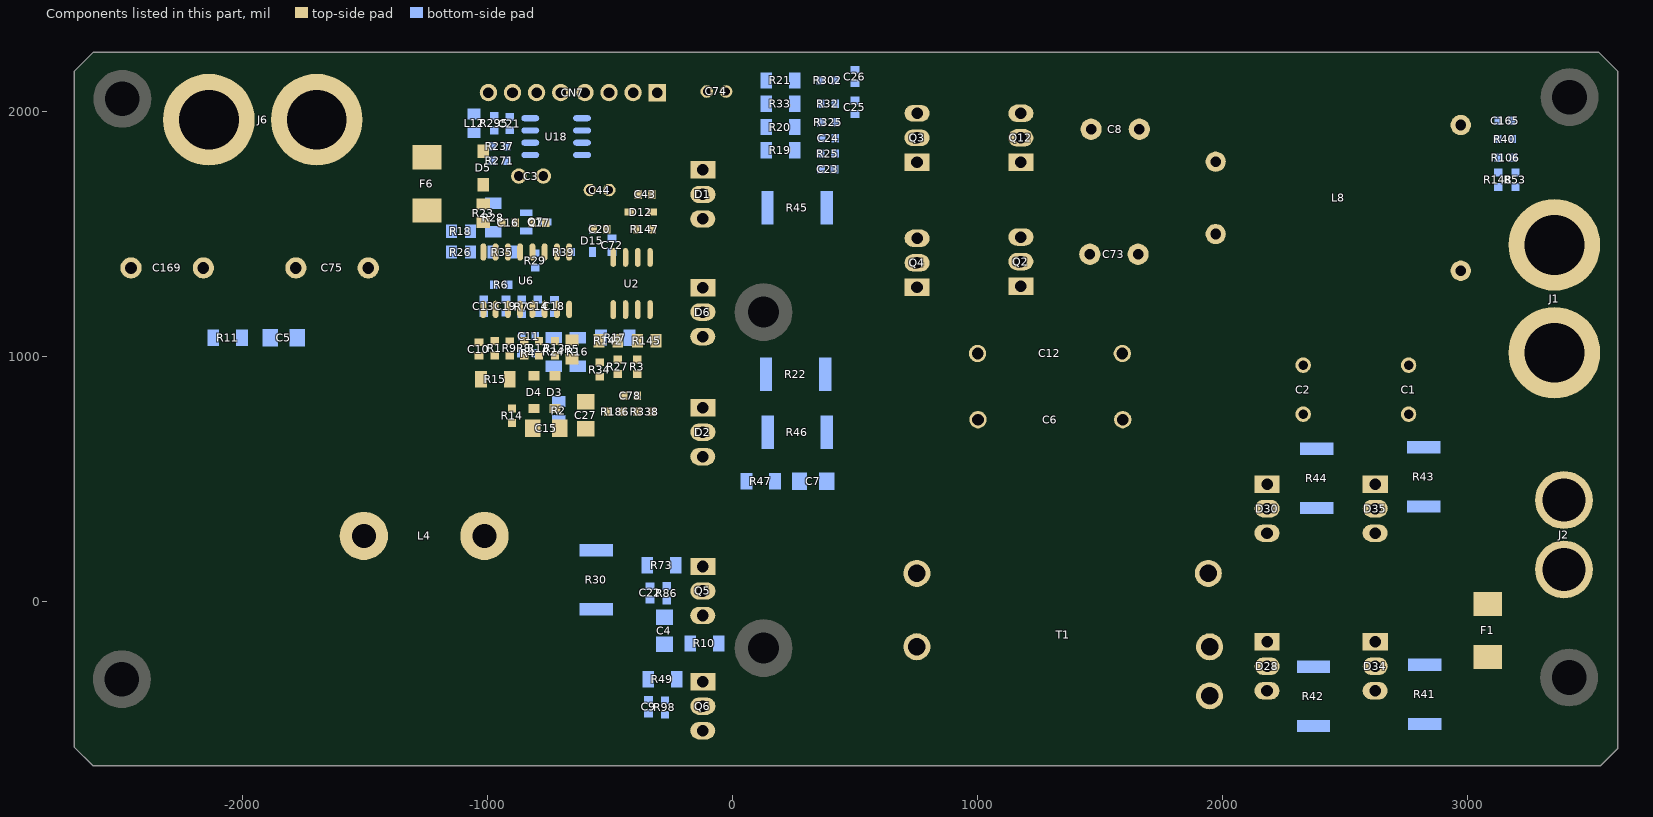
[diagram p0: the components of this part, seen from the top]
# Altium PCB MISC89356.PcbDoc (part 3 of 3)
Units mil, origin at the board's own origin, x right, y up, seen from the top; angles counter-clockwise.
Board outline 6299.21 x 2912.91 mil, 4 copper layers (Top Layer, GND02, PWR03, Bottom Layer); 128 components, 68 nets, 313 pads, 200 vias.

## Polygon pours and split planes (outlines as drawn) (continued)
GND on GND02 "Bottom Layer-No Net 2" (solid, remove dead copper, pour order 1001): -1142.15,2154.47 -1142.15,779.66 -897.15,527.35 -877.15,506.76 -877.15,-239.86 -877.15,-569.4 -897.15,-590 -2607.15,-590 -2687.15,-507.61 -2687.15,2159.61 -2607.15,2242 -1152.15,2242 -1147.15,2236.85 -1142.15,2231.7 -1142.15,2154.47
BAT- on GND02 "BottomLayer-No Net" (solid, remove dead copper, pour order 1004): -653,89 -653,72 -653,-517 -607,-563 -591,-579 -132,-579 557,-579 619,-517 654,-482 654,-413 654,779 675,800 683,808 865,808 1746,808 1813,741 1854,700 1854,29 1854,-451 1877,-474 1927,-524 2014,-524 3513,-524 3555,-482 3581,-456 3581,-411 3581,1604 3545,1640 3523,1662 3447,1662 2997,1662 2954,1619 2932,1597 2932,1455 2932,1188 2870,1126 2862,1118 2796,1118 1825,1118 1778,1165 1758,1185 1758,1326 1758,2097 1688,2167 1668,2187 1585,2187 292,2187 239,2134 227,2122 227,2090 227,1802 209,1784 204,1779 142,1779 -140,1779 -204,1715 -231,1688 -231,1584 -231,212 -254,189 -256,191 -533,191 -600,191 -639,152 -653,138 -653,90
GND on GND02 "BottomLayer-No Net" (solid, remove dead copper, pour order 1006): -1061,2137 -1061,838 -807,584 -684,461 -684,300 -684,293 -664,273 -649,258 -585,258 -364,258 -344,278 -339,283 -339,743 -339,815 -315,839 -298,856 -298,902 -298,1836 -267,1867 -259,1875 -36,1875 24,1875 58,1909 69,1920 69,1975 69,2161 44,2186 23,2207 -30,2207 -994,2207 -1062,2139
NetD30_1 on PWR03 "BottomLayer-No Net" (solid, remove dead copper, pour order 1004): 1869,318 1869,93 1898,64 1904,58 1917,45 2667,45 2746,45 2780,79 2805,104 2805,211 2805,555 2748,612 2723,637 2651,637 1943,637 1893,587 1869,563 1869,318
NetD28_1 on PWR03 "BottomLayer-No Net" (solid, remove dead copper, pour order 1003): 1883,-339 1883,-461 1898,-476 1913,-491 1942,-491 2742,-491 2767,-466 2777,-456 2777,-389 2777,-84 2750,-57 2730,-37 2681,-37 2104,-37 2053,-88 2043,-98 2043,-165 2043,-234 2019,-258 1998,-279 1945,-279 1899,-279 1891,-287 1883,-295 1883,-339
GND on PWR03 "Bottom Layer-No Net 2" (solid, remove dead copper, pour order 1006): -1142.15,2154.74 -1142.15,784.31 -897.15,532.8 -877.15,512.27 -877.15,-231.97 -877.15,-560.47 -897.15,-581 -2607.15,-581 -2687.15,-498.88 -2687.15,2159.88 -2607.15,2242 -1152.15,2242 -1147.15,2236.87 -1142.15,2231.73 -1142.15,2154.74
BAT- on PWR03 "BottomLayer-No Net" (solid, remove dead copper, pour order 1008): -683,-31 -683,-523 -651,-555 -597,-609 -216,-609 577,-609 623,-563 649,-537 649,-367 649,715 719,785 800,866 2364,866 2839,866 2928,777 3003,702 3003,517 3003,380 3044,339 3122,261 3342,261 3476,261 3522,307 3570,355 3570,495 3570,1785 3527,1828 3514,1841 3337,1841 3118,1841 3085,1808 3068,1791 3068,1535 3068,1129 3048,1109 3040,1101 2835,1101 1871,1101 1843,1129 1829,1143 1829,1369 1829,2108 1773,2164 1749,2188 1660,2188 260,2188 241,2169 233,2161 233,2113 233,1865 209,1841 177,1809 -31,1809 -166,1809 -181,1794 -224,1751 -224,1725 -224,181 -267,138 -313,92 -538,92 -636,92 -672,56 -683,45 -683,-30
GND on PWR03 "BottomLayer-No Net" (solid, remove dead copper, pour order 1009): -1060,2162 -1060,851 -723,514 -713,504 -713,439 -713,299 -679,265 -662,248 -590,248 -366,248 -343,271 -343,727 -343,835 -308,870 -298,880 -298,918 -298,1817 -248,1867 -232,1883 -70,1883 44,1883 78,1917 86,1925 86,1988 86,2158 53,2191 36,2208 -20,2208 -1022,2208 -1056,2174 -1060,2170 -1060,2162
NetC1_1 on Bottom Layer "BottomLayer-No Net" (solid, remove dead copper, pour order 1006): 2212,803 2212,634 2242,604 2263,583 2348,583 2877,583 2922,538 2968,492 2968,-81 2968,-368 2916,-420 2901,-435 2558,-435 2314,-435 2300,-449 2292,-457 2292,-482 2292,-550 2297,-555 2314,-572 2347,-572 3041,-572 3084,-529 3172,-441 3172,-84 3172,751 3112,811 3070,853 2740,853 2231,853 2212,834 2212,804
NetD30_2 on Bottom Layer "BOTTOM-No Net" (solid, remove dead copper, pour order 1004): 2403.36,183 2091.47,183 2074.15,204.6 2074.15,415.2 2082.81,426 2455.34,426 2464,415.2 2464,199.2 2455.34,188.4 2451,183 2403.36,183
LLC_I on Bottom Layer "BottomLayer-No Net" (solid, remove dead copper, pour order 1005): 569,517 569,497 569,97 604,62 617,49 688,49 786,49 799,62 809,72 809,122 809,574 862,627 875,640 967,640 1038,640 1061,663 1085,687 1085,732 1085,1061 1072,1074 1050,1096 992,1096 765,1096 689,1020 569,900 569,517
NetD35_2 on Bottom Layer "BOTTOM-No Net" (solid, remove dead copper, pour order 1005): 2567.53,419 2884.06,419 2907,393.4 2907,183.48 2888.65,163 2553.76,163 2540,178.36 2540,408.76 2549.18,419 2567.53,419
NetD28_2 on Bottom Layer "BOTTOM-No Net" (solid, remove dead copper, pour order 1006): 2053.85,-38 2423.85,-38 2443.85,-58 2443.85,-288 2428.85,-303 2068.85,-303 2038.85,-273 2038.85,-53
NetD34_2 on Bottom Layer "BOTTOM-No Net" (solid, remove dead copper, pour order 1007): 2566.29,-45 2886.23,-45 2904,-65 2904,-280 2890.67,-295 2886.23,-300 2597.39,-300 2530.74,-300 2521.85,-290 2521.85,-60 2535.18,-45 2566.29,-45
NetD1_2 on Bottom Layer "Bottom Layer-No Net 2" (solid, remove dead copper, pour order 1008): 187.85,1472 187.85,1702 172.85,1717 37.85,1717 22.85,1732 22.85,1827 2.85,1847 -222.15,1847 -232.15,1837 -232.15,1442 -212.15,1422 172.85,1422 187.85,1437 187.85,1472
PV+ on Bottom Layer "Bottom Layer-No Net 2" (solid, remove dead copper, pour order 1009): -1247.15,2147 -1212.15,2112 -1212.15,1747 -1232.15,1727 -1847.15,1727 -1862.15,1742 -1862.15,2062 -1777.15,2147
GND on Bottom Layer "Bottom Layer-No Net 2" (solid, remove dead copper, pour order 1011): -466.15,349 -661.15,349 -676.15,334 -676.15,144 -656.15,124 -411.15,124 -396.15,139 -396.15,279 -466.15,349
GND on Bottom Layer "Bottom Layer-No Net 2" (solid, remove dead copper, pour order 1012): -1142.15,2154.47 -1142.15,779.66 -897.15,527.35 -877.15,506.76 -877.15,-239.86 -877.15,-569.4 -897.15,-590 -2607.15,-590 -2687.15,-507.61 -2687.15,2159.61 -2607.15,2242 -1152.15,2242 -1147.15,2236.85 -1142.15,2231.7 -1142.15,2154.47
BAT- on Bottom Layer "BottomLayer-No Net" (solid, remove dead copper, pour order 1012): -687,-31 -687,-507 -636,-558 -583,-611 -179,-611 -91,-611 -65,-585 -61,-581 -61,-545 -61,-511 -77,-495 -85,-487 -110,-487 -199,-487 -219,-467 -242,-444 -271,-444 -368,-444 -398,-414 -412,-400 -412,-239 -412,12 -425,25 -434,34 -465,34 -668,34 -681,21 -687,15 -687,-31
NetD6_2 on Bottom Layer "BottomLayer-No Net" (solid, remove dead copper, pour order 1013): -129,1231 -220,1231 -259,1192 -265,1186 -265,1107 -265,979 -227,941 -217,931 -77,931 -20,931 46,865 58,853 148,853 169,853 188,872 193,877 193,937 193,1005 172,1026 161,1037 114,1037 31,1037 -6,1074 -24,1092 -24,1185 -24,1200 -43,1219 -55,1231 -128,1231
NetD2_2 on Bottom Layer "BottomLayer-No Net" (solid, remove dead copper, pour order 1014): -253,831 -253,708 -231,686 -198,653 -124,653 6,653 37,622 54,605 115,605 167,605 182,620 200,638 200,679 200,788 178,810 176,812 126,812 44,812 -16,872 -34,890 -97,890 -227,890 -244,873 -253,864 -253,832
NetC7_2 on Bottom Layer "BottomLayer-No Net" (solid, remove dead copper, pour order 1015): 347,891 347,457 304,414 282,392 112,392 30,392 -50,472 -74,496 -150,496 -255,496 -325,566 -381,622 -381,955 -381,1107 -388,1114 -390,1116 -407,1116 -437,1116 -445,1108 -452,1101 -452,1068 -452,627 -283,458 -255,430 -145,430 -90,430 -25,365 22,318 213,318 386,318 449,381 490,422 490,596 490,983 567,1060 652,1145 796,1145 1499,1145 1541,1187 1571,1217 1571,1391 1571,2017 1560,2028 1545,2043 1502,2043 1344,2043 1334,2033 1302,2001 1302,1968 1302,1761 1278,1737 1232,1691 470,1691 379,1691 365,1677 347,1659 347,890

## Keep-outs
Keep-Out Layer:
  circle w10: c3414.78,2059.05 r70.87
  circle w10: c3412.93,-309.1 r70.87
  circle w10: c-2492.15,-315.95 r70.87
  circle w10: c-2490.3,2052.2 r70.87
  lines w25: -2687.15,-592 -2687.15,2164.17 -2608.41,2242.91 3533.33,2242.91 3612.07,2164.17 3612.07,-597.79 3539.85,-670 -2609.15,-670 -2687.15,-592

## Other copper
Top Layer:
  rectangle net NetD1_1: -231.15,-461 -21.15,-391
  rectangle net NetD1_1: -201.15,9 -26.15,79
  rectangle net NetD1_1: -207.15,762 -37.15,822
  rectangle net NetD1_1: -162.15,787 -82.15,857
  rectangle net NetD1_1: -162.54,527 -82.54,597
  rectangle net NetD1_1: -207.54,562 -37.54,622
  rectangle net NetD1_1: -207.15,1252 -37.15,1312
  rectangle net NetD1_1: -162.15,1277 -82.15,1347
  rectangle net NetD1_1: -162.54,1017 -82.54,1087
  rectangle net NetD1_1: -207.54,1052 -37.54,1112
  rectangle net NetD1_1: -207.54,1532 -37.54,1592
  rectangle net NetD1_1: -162.54,1497 -82.54,1567
  rectangle net NetD1_1: -162.15,1757 -82.15,1827
  rectangle net NetD1_1: -207.15,1732 -37.15,1792
  rectangle net T1H: 1095.46,1458 1265.46,1518
  rectangle net T1H: 1145.46,1488 1225.46,1558
  rectangle net T1H: 721.85,1482 801.85,1552
  rectangle net T1H: 671.85,1452 841.85,1512
  rectangle net T1H: 1935.85,1733 2005.85,1863
  rectangle net T1H: 1895.85,1763 2050.85,1833
  rectangle net NetL8_4: 700.85,-270 795.85,-90
  rectangle net NetL8_4: 661.85,-230 836.85,-135
  rectangle net NetL8_4: 1940.85,1438 2005.85,1568
  rectangle net NetL8_4: 1900.85,1472 2045.85,1532
  rectangle net GND: -633.71,1665 -583.71,1700
  rectangle net GND: -598.71,1630 -563.71,1730
  rectangle net +12V: -520.71,1384 -485.71,1431.2
  rectangle net +12V: -513.71,1659.53 -458.71,1700
  rectangle net +12V: -523.71,1625 -483.71,1730
  rectangle net GND: -2349,1857 -1947.15,2077
  rectangle net GND: -2277.15,1737 -1997.15,2182
  rectangle net PV+: -1901.15,1827 -1446.15,2113
  rectangle net PV+: -1809.15,1735 -1590.15,2177
  rectangle net PV+: -1382.15,1722 -1143.09,1854
  rectangle net PV+: -1297.15,1737 -1197.15,1927
  rectangle net PV-OVP: -1170.15,205 -863.15,340
  rectangle net PV-OVP: -1074.15,110 -946.15,410
  rectangle net PV-OVP: -1878.15,1329 -1686.15,1397
  rectangle net PV-OVP: -1813.15,1263 -1752.15,1449
  rectangle net PV-OVP: -2543.06,1329 -2358.15,1393
  rectangle net PV-OVP: -2485.15,1257 -2421.15,1463
  rectangle net PV-OVP: -1366.15,1561 -1142.15,1633
  rectangle net PV-OVP: -1293.15,1472 -1197.15,1577
  rectangle net NetC1_1: 2237.85,742 2417.85,792
  rectangle net NetC1_1: 2302.85,687 2352.85,847
  rectangle net NetC1_1: 2732.85,687 2782.85,847
  rectangle net NetC1_1: 2667.85,742 2847.85,792
  rectangle net +12V: -797.15,1677 -747.15,1807
  rectangle net +12V: -737.66,2007 -667.15,2077.45
  rectangle net NetD1_1: -1678.15,198.84 -1373.15,340
  rectangle net NetD1_1: -1583.15,125 -1423.15,395
  pour cut-out: -1540.15,1273 -1432.15,1273 -1432.15,1203 -1540.15,1203
  pour cut-out: 3037.23,2181.62 3050.85,2168 3050.85,1178 3030.85,1158 2216.27,1158 2201.27,1173 2205.85,2178 2210.85,2183
  pour cut-out: -2261.15,1293.93 -2139.08,1293.93 -2127.15,1282 -2127.15,1192 -2132.15,1187 -2266.47,1187 -2272.47,1193 -2272.47,1282.61
GND02:
  rectangle net GND: -1516.49,1283 -1460.49,1439
  rectangle net GND: -1557.49,1331 -1405.49,1394
  rectangle net GND: -2230.15,1331 -2078.15,1394
  rectangle net GND: -2189.15,1283 -2133.15,1439
  rectangle net GND: -2265.15,1732 -2025.15,2182
  rectangle net GND: -2350,1857 -1922.15,2082
  rectangle net GND: -1192.15,1412 -1027.15,1527
  rectangle net GND: -822.15,2012 -772.15,2147
  rectangle net GND: -897.15,1677 -847.15,1797
  rectangle net GND: -942.15,1717 -882.15,1757
  rectangle net GND: -603.71,1625 -562.15,1737
  rectangle net GND: -642.15,1662 -582.15,1697
  rectangle net BAT-: 2247.85,937 2407.85,992
  rectangle net BAT-: 2302.85,882 2352.85,1052
  rectangle net BAT-: 2732.85,882 2782.85,1052
  rectangle net BAT-: 2677.85,937 2837.85,992
  pour cut-out: 2824.23,2175.62 2837.85,2162 2837.85,1172 2817.85,1152 2003.27,1152 1988.27,1167 1992.85,2172 1997.85,2177
PWR03:
  rectangle net GND: -2252.15,1727 -2037.15,2181
  rectangle net GND: -2357.15,1867 -1924.64,2073
  rectangle net GND: -2181.15,1287 -2133.15,1432
  rectangle net GND: -2242.15,1332 -2085.15,1388.25
  rectangle net GND: -1509.15,1287 -1461.15,1432
  rectangle net GND: -1557.15,1337 -1407.15,1392
  rectangle net NetD28_1: 2094.85,-197 2264.85,-137
  rectangle net NetD28_1: 2129.85,-167 2224.85,-107
  rectangle net NetD28_1: 2570.85,-166 2665.85,-106
  rectangle net NetD28_1: 2535.85,-196 2705.85,-136
  region net NetD28_1: 2229.46,-367 2134.46,-367 2134.46,-427 2229.46,-427
  region net NetD28_1: 2264.46,-337 2094.46,-337 2094.46,-397 2264.46,-397
  region net NetD28_1: 2670.46,-366 2575.46,-366 2575.46,-426 2670.46,-426
  region net NetD28_1: 2705.46,-336 2535.46,-336 2535.46,-396 2705.46,-396
  rectangle net BAT-: 2677.85,937 2837.85,992
  rectangle net BAT-: 2732.85,882 2782.85,1052
  rectangle net BAT-: 2302.85,882 2352.85,1052
  rectangle net BAT-: 2247.85,937 2407.85,992
  rectangle net GND: -827.15,2002 -772.15,2147
  pour cut-out: 2824.23,2175.62 2837.85,2162 2837.85,1172 2817.85,1152 2003.27,1152 1988.27,1167 1992.85,2172 1997.85,2177
Bottom Layer:
  rectangle net NetD1_2: 52.85,1489.5 187.85,1702
  rectangle net NetD1_2: -202.15,1627 -32.15,1692
  rectangle net LLC_I: 964.85,952 1019.85,1077
  rectangle net LLC_I: 935.85,990 1055.85,1045
  rectangle net GND: -2181.15,1282 -2127.15,1437
  rectangle net GND: -2229.15,1341 -2087.15,1387
  rectangle net GND: -1521.15,1292 -1449.15,1437
  rectangle net GND: -1548.38,1337 -1413.15,1387
  rectangle net GND: -2257.15,1713 -2012.15,2182
  rectangle net GND: -2349.15,1887 -1929.15,2077
  region net NetD30_2: 2459,417 2132,417 2132,347 2459,347
  rectangle net NetD35_2: 2585.85,346 2894,416
  region net NetD28_2: 2432,-226.7 2131,-226.7 2131,-296.7 2432,-296.7
  rectangle net NetD34_2: 2581.85,-295 2895,-225
  rectangle net NetC1_1: 2227.85,737 2412.85,792
  rectangle net NetC1_1: 2302.85,672 2347.85,847
  rectangle net NetC1_1: 2732.85,672 2777.85,847
  rectangle net NetC1_1: 2657.85,737 2842.85,792
  rectangle net PV+: -1687.15,1792 -1402.15,2147
  rectangle net PV+: -1862.15,1742 -1522.15,1937
  rectangle net BAT-: -670.71,-131 -426.15,19
  rectangle net LLC_I: 939.85,717 1059.85,772
  rectangle net LLC_I: 968.85,679 1023.85,804
  pour cut-out: 2899.23,2175.62 2912.85,2162 2912.85,1172 2892.85,1152 2078.27,1152 2063.27,1167 2067.85,2172 2072.85,2177

## Silkscreen, mask and mechanical layers (free items; w line width, h text height)
Top Overlay:
  rectangle: 118,-640 394,1391
  lines w5: -865.15,858.69 -865.15,873.69 -844.25,873.69
Bottom Overlay:
  lines w5: -855.15,1149.5 -855.15,1130 -535,1130 -535,1289 -855.15,1289 -855.15,1258.57
outline:
  circle w5: c-2490.3,2052.2 r70.87
  circle w5: c-2492.15,-315.95 r70.87
  circle w5: c3412.93,-309.1 r70.87
  circle w5: c3414.78,2059.05 r70.87
  lines w5: -2687.15,-591.26 -2614.06,-664.35 -2607.93,-670.48 3533.37,-670.48 3612.07,-591.79 3612.07,2164.17 3533.33,2242.91 -2608.41,2242.91 -2687.15,2164.17 -2687.15,-591.26
Mechanical 2:
  lines w10: -1299.51,-1928 -1299.51,4367 ; 46.91,-588 46.91,2372 ; 637.46,-583 637.46,2377 ; 876.71,-1683 876.71,4537
  text "No tall components in the middle" at -871.4,3187 h40
  text "Input" at -2197.15,2567 h40
  text "Output" at 2207.85,2512 h40
Mechanical 15:
  lines w0.1: -1795.8,336.42 -1795.82,336.44 ; 265.91,726.56 265.89,726.58 ; 265.91,1103.56 265.89,1103.58 ; 847.63,1152.41 847.61,1152.43 ; 889.91,1506.56 889.89,1506.58 ; 1491.62,1666.2 1491.64,1666.22 ; 1581.7,490.22 1581.72,490.24 ; -2212.16,1616.99 -2212.14,1617.01
Drill Drawing:
  text ".Legend" at 4508.85,3 h40

## Dimensions
-1299.51,4367 to 863.6,3137 on Mechanical 2
3552.85,2242.91 to 3542.85,-513 on Drill Drawing
-2687.15,2164.17 to 3612.07,2164.17 on Drill Drawing